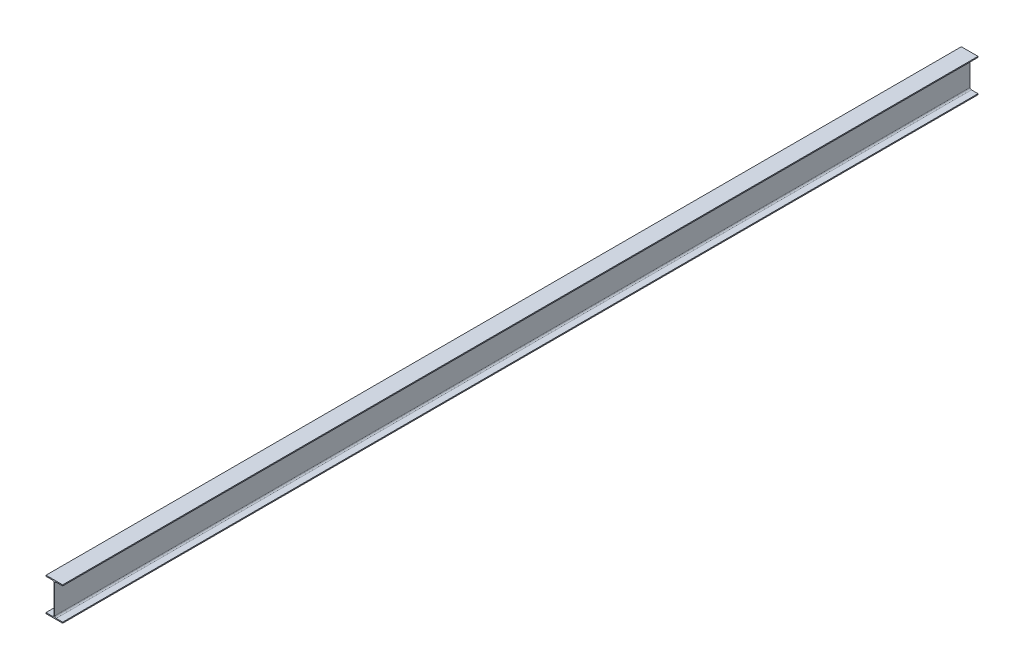
SolidWorks part; units mm, degrees
ref_plane "Front Plane" through (0, 0, 0) normal (0, 0, 1) x (1, 0, 0)
ref_plane "Top Plane" through (0, 0, 0) normal (0, 1, 0) x (1, 0, 0)
ref_plane "Right Plane" through (0, 0, 0) normal (1, 0, 0) x (0, 0, -1)
other "Configuration Table"
sketch "Sketch1" plane through (0, 0, 0) normal (0, 0, 1) x (1, 0, 0)
  line L0 (0, 0) -> (0, 300) construction
  line L1 (75, 0) -> (-75, 0)
  line L2 (-75, 0) -> (-75, 9)
  line L3 (-75, 9) -> (-16.25, 9)
  line L4 (3.25, 22) -> (3.25, 278)
  line L6 (-75, 291) -> (-75, 300)
  line L7 (-75, 300) -> (75, 300)
  line L8 (-3.25, 22) -> (-3.25, 278)
  line L9 (75, 291) -> (75, 300)
  line L10 (16.25, 291) -> (75, 291)
  line L11 (75, 9) -> (16.25, 9)
  line L12 (75, 0) -> (75, 9)
  line L13 (-16.25, 291) -> (-75, 291)
  arc A0 (16.25, 9) -> (3.25, 22) centre (16.25, 22) cw
  arc A1 (-3.25, 22) -> (-16.25, 9) centre (-16.25, 22) cw
  arc A2 (3.25, 278) -> (16.25, 291) centre (16.25, 278) cw
  arc A3 (-3.25, 278) -> (-16.25, 291) centre (-16.25, 278) ccw
  point P18 (3.25, 9)
  point P21 (-3.25, 9)
  point P24 (3.25, 291)
  point P27 (-3.25, 291)
  dimension "D6" = 13
  dimension "D1" = 300
  dimension "D2" = 150
  dimension "D3" = 6.5
  dimension "D4" = 9
  dimension "D5" = 9
extrude "Boss-Extrude1" add sketch "Sketch1" along normal blind 8240
